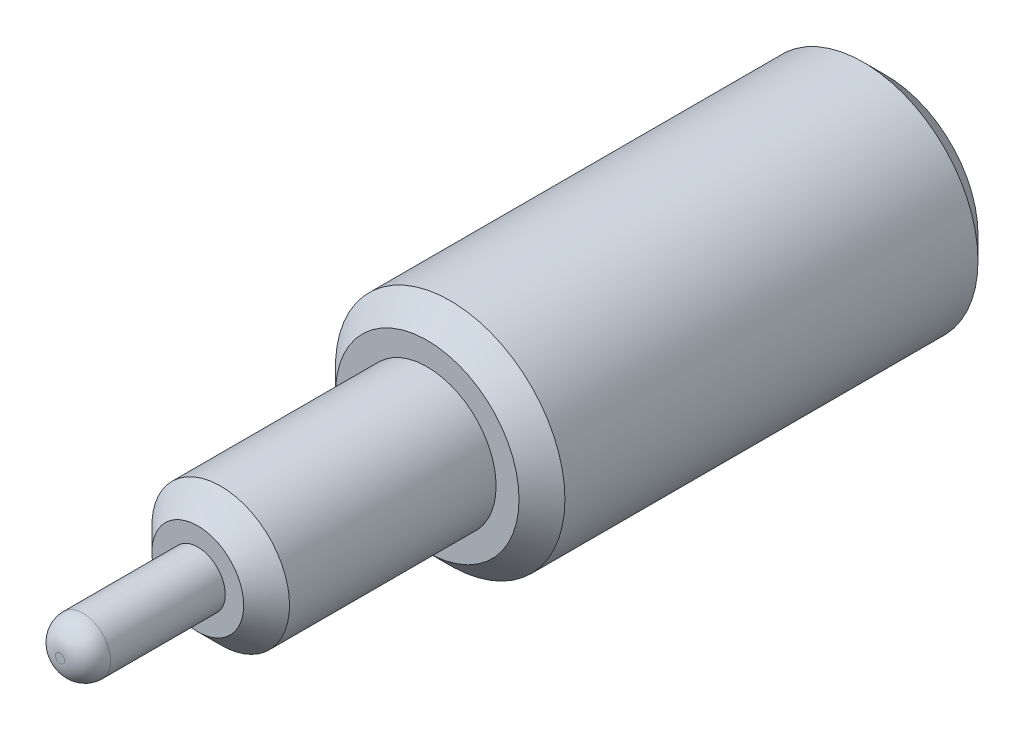
SolidWorks part; units mm, degrees
ref_plane "Front Plane" through (0, 0, 0) normal (0, 0, 1) x (1, 0, 0)
ref_plane "Top Plane" through (0, 0, 0) normal (0, 1, 0) x (1, 0, 0)
ref_plane "Right Plane" through (0, 0, 0) normal (1, 0, 0) x (0, 0, -1)
other "Configuration Table"
sketch "Sketch1" plane through (0, 0, 0) normal (0, 0, 1) x (1, 0, 0)
  circle A0 centre (0, 0) radius 2.5
  dimension "D1" = 5
extrude "Boss-Extrude1" add sketch "Sketch1" along normal blind 10
sketch "Sketch2" plane through (0, 0, 10) normal (0, 0, 1) x (1, 0, 0)
  circle A0 centre (0, 0) radius 1.5
  dimension "D1" = 3
extrude "Boss-Extrude2" add sketch "Sketch2" along normal blind 5
sketch "Sketch3" plane through (0, 0, 15) normal (0, 0, 1) x (1, 0, 0)
  circle A0 centre (0, 0) radius 0.6
  dimension "D1" = 1.2
extrude "Boss-Extrude3" add sketch "Sketch3" along normal blind 3
fillet "Fillet1" radius 0.5 1 edges at (0.6, 0, 18)
sketch "Sketch4" plane through (0, 0, 0) normal (0, 0, -1) x (-1, 0, 0)
  circle A0 centre (0, 0) radius 0.8924
extrude "Cut-Extrude1" cut sketch "Sketch4" against normal blind 13
chamfer "Chamfer1" distance 0.5 angle 45 3 edges at (1.5, 0, 15) (2.5, 0, 10) (2.5, 0, 0)
